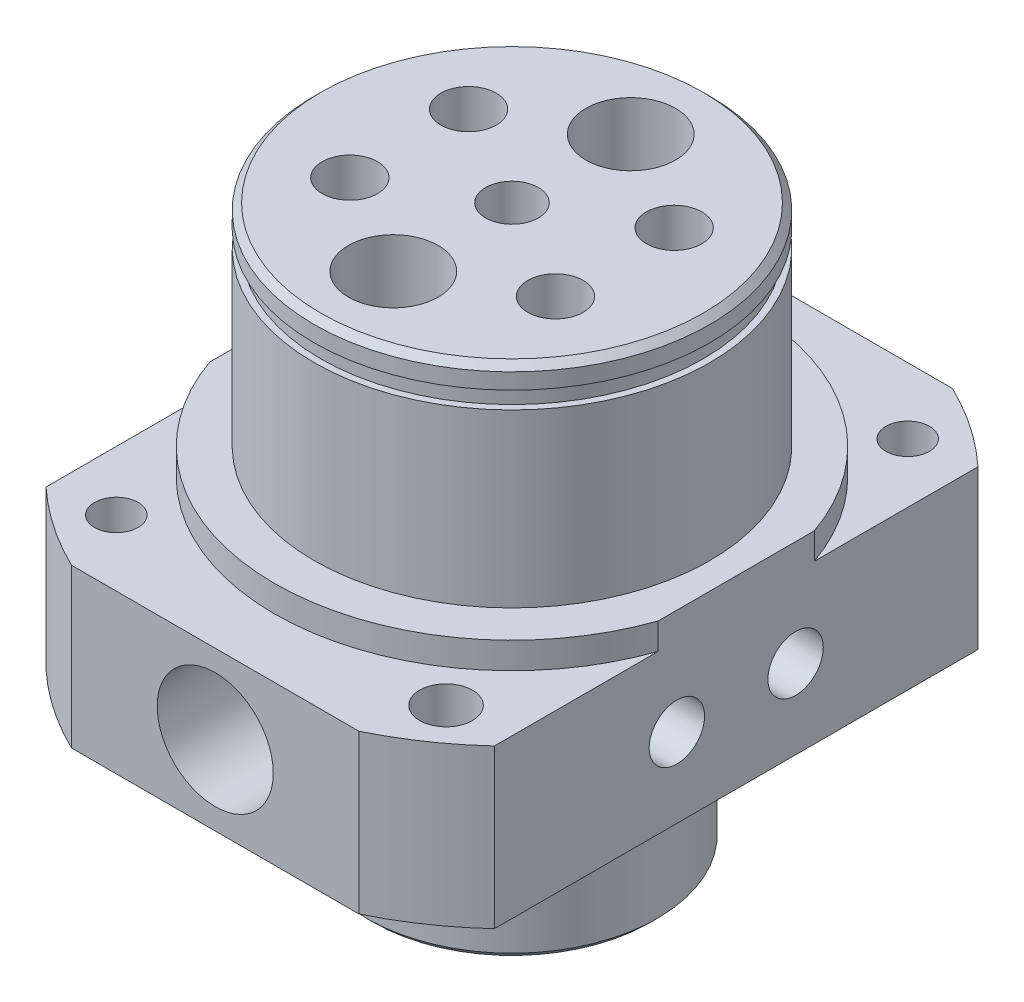
SolidWorks part; units mm, degrees
material "S45C"
ref_plane "Front Plane" through (0, 0, 0) normal (0, 0, 1) x (1, 0, 0)
ref_plane "Top Plane" through (0, 0, 0) normal (0, 1, 0) x (1, 0, 0)
ref_plane "Right Plane" through (0, 0, 0) normal (1, 0, 0) x (0, 0, -1)
sketch "Sketch1" plane through (0, 0, 0) normal (1, 0, 0) x (0, 0, -1)
  line L0 (0, 78.7622) -> (0, -44.4545) construction
  line L1 (0, -12) -> (11, -12)
  line L2 (11, -12) -> (11, 0)
  line L3 (11, 0) -> (25, 0)
  line L4 (25, 0) -> (25, 12)
  line L5 (25, 12) -> (18, 12)
  line L6 (15, 14) -> (15, 27)
  line L7 (15, 30) -> (0, 30)
  line L8 (0, 30) -> (0, -12)
  line L9 (18, 12) -> (18, 14)
  line L10 (18, 14) -> (15, 14)
  line L11 (15, 28.3) -> (14.5, 28.3)
  line L12 (14.5, 28.3) -> (14.5, 27)
  line L13 (14.5, 27) -> (15, 27)
  line L14 (15, 28.3) -> (15, 30)
  dimension "D1" = 11
  dimension "D2" = 25
  dimension "D3" = 15
  dimension "D4" = 12
  dimension "D5" = 12
  dimension "D6" = 13
  dimension "D7" = 18
  dimension "D8" = 2
  dimension "D9" = 14.5
  dimension "D10" = 1.3
  dimension "D11" = 1.7
revolve "Revolve1" add sketch "Sketch1" angle 360 about L0
sketch "Sketch2" plane through (0, 0, 0) normal (0, 1, 0) x (1, 0, 0)
  line L1 (-17, -22.5) -> (17, -22.5)
  line L2 (-17, -22.5) -> (-17, 22.5)
  line L3 (-17, 22.5) -> (17, 22.5)
  line L4 (17, -22.5) -> (17, 22.5)
  line L5 (-17, -22.5) -> (17, 22.5) construction
  line L6 (-17, 22.5) -> (17, -22.5) construction
  point P0 (0, 0)
  dimension "D1" = 34
  dimension "D2" = 45
extrude "Cut-Extrude1" cut sketch "Sketch2" along normal through all flip side to cut
sketch "Sketch3" plane through (0, -12, 0) normal (0, -1, 0) x (1, 0, 0)
  circle A0 centre (0, 0) radius 5.5
  dimension "D1" = 11
extrude "Cut-Extrude2" [suppressed] cut sketch "Sketch3" against normal through all
hole_wizard "M4 Tapped Hole1" positions "Sketch13" profile "Sketch12" tap size "M4" standard "Gb" end condition through all
sketch "Sketch13" plane through (0, 0, 0) normal (0, -1, 0) x (-1, 0, 0)
  line L1 (-12.5, -17.5) -> (12.5, -17.5) construction
  line L2 (-12.5, -17.5) -> (-12.5, 17.5) construction
  line L3 (-12.5, 17.5) -> (12.5, 17.5) construction
  line L4 (12.5, -17.5) -> (12.5, 17.5) construction
  line L5 (-12.5, -17.5) -> (12.5, 17.5) construction
  line L6 (-12.5, 17.5) -> (12.5, -17.5) construction
  point P0 (-12.5, 17.5)
  point P2 (12.5, -17.5)
  dimension "D1" = 35
  dimension "D2" = 25
sketch "Sketch12" plane through (12.5, 0, -17.5) normal (1, 0, 0) x (0, 0, -1)
  line L0 (0, 0) -> (0, 30)
  line L1 (0, 30) -> (1.65, 30)
  line L2 (1.65, 30) -> (1.65, 0)
  line L5 (1.65, 0) -> (0, 0)
  line L11 (0, -6.35) -> (0, 107.95) construction
  dimension "通孔螺纹孔钻头直径" = 3.3
  dimension "通孔螺纹孔钻头深度" = 30
cosmetic thread "Cosmetic Thread8" parameters "D2"=4
cosmetic thread "Cosmetic Thread11" parameters "D2"=4
sketch "Sketch14" plane through (0, 12, 0) normal (0, 1, 0) x (1, 0, 0)
  line L1 (12.5, -17.5) -> (-12.5, -17.5) construction
  line L2 (12.5, -17.5) -> (12.5, 17.5) construction
  line L3 (12.5, 17.5) -> (-12.5, 17.5) construction
  line L4 (-12.5, -17.5) -> (-12.5, 17.5) construction
  line L5 (12.5, -17.5) -> (-12.5, 17.5) construction
  line L6 (12.5, 17.5) -> (-12.5, -17.5) construction
  circle A0 centre (12.5, -17.5) radius 2
  circle A1 centre (-12.5, 17.5) radius 2
  point P2 (0, 0)
  dimension "D1" = 4
extrude "Cut-Extrude5" cut sketch "Sketch14" against normal through all
sketch "Sketch15" plane through (17, 0, 0) normal (1, 0, 0) x (0, 0, -1)
  line L0 (-3, 6) -> (3, 6) construction
  line L1 (-3, 9) -> (3, 9)
  line L2 (-3, 3) -> (3, 3)
  line L3 (22.5, 6) -> (-22.5, 6) construction
  line L4 (22.5, 12) -> (22.5, 0) construction
  line L5 (-22.5, 0) -> (-22.5, 12) construction
  arc A0 (-3, 9) -> (-3, 3) centre (-3, 6) ccw
  arc A1 (3, 3) -> (3, 9) centre (3, 6) ccw
  point P2 (0, 6)
  dimension "D2" = 3
  dimension "D1" = 6
extrude "Cut-Extrude6" [suppressed] cut sketch "Sketch15" against normal through all
sketch "Sketch17" plane through (0, 30, 0) normal (0, 1, 0) x (1, 0, 0)
  line L0 (0, -30.9464) -> (0, 32.404) construction
  line L1 (-7.7942, 4.5) -> (7.7942, -4.5) construction
  line L2 (7.7942, 4.5) -> (-7.7942, -4.5) construction
  circle A0 centre (-7.7942, 4.5) radius 2
  circle A1 centre (-7.7942, -4.5) radius 2
  circle A2 centre (0, -9) radius 3
  circle A3 centre (7.7942, 4.5) radius 2
  circle A4 centre (0, 9) radius 3
  circle A5 centre (7.7942, -4.5) radius 2
  circle A6 centre (0, 0) radius 2
  circle A7 centre (0, 0) radius 9 construction
  dimension "D1" = 6
  dimension "D2" = 4
  dimension "D3" = 4
  dimension "D4" = 18
  dimension "D5" = 60
  dimension "D6" = 60
extrude "Cut-Extrude7" cut sketch "Sketch17" against normal blind 28
sketch "Sketch18" plane through (-17, 0, 0) normal (-1, 0, 0) x (0, 0, 1)
  line L0 (0, 0) -> (0, 38.293) construction
  line L1 (-18.3303, 0) -> (18.3303, 0) construction
  circle A0 centre (-4.5, 6) radius 2
  circle A1 centre (4.5, 6) radius 2
  dimension "D1" = 9
  dimension "D2" = 6
  dimension "D3" = 4
extrude "Cut-Extrude10" cut sketch "Sketch18" against normal up to next
sketch "Sketch19" plane through (17, 0, 0) normal (1, 0, 0) x (0, 0, -1)
  circle A0 centre (-4.5, 6) radius 2
  circle A1 centre (4.5, 6) radius 2
  dimension "D1" = 4
extrude "Cut-Extrude11" cut sketch "Sketch19" against normal up to next
sketch "Sketch20" plane through (0, 0, -22.5) normal (0, 0, -1) x (-1, 0, 0)
  line L0 (-10.8972, 0) -> (10.8972, 0) construction
  circle A0 centre (0, 6) radius 3
  dimension "D1" = 6
  dimension "D2" = 6
extrude "Cut-Extrude12" cut sketch "Sketch20" against normal up to next
sketch "Sketch21" plane through (0, 0, 22.5) normal (0, 0, 1) x (1, 0, 0)
  circle A0 centre (0, 6) radius 3
  dimension "D1" = 6
extrude "Cut-Extrude13" cut sketch "Sketch21" against normal up to next
sketch "Sketch22" plane through (0, -12, 0) normal (0, -1, 0) x (1, 0, 0)
  circle A0 centre (0, 0) radius 2
  dimension "D1" = 4
extrude "Cut-Extrude14" cut sketch "Sketch22" against normal through all
chamfer "Chamfer1" distance 0.5 angle 45 2 edges at (0, -12, 11) (0, 30, 15)
chamfer "Chamfer2" [suppressed] distance 0.5 angle 45
hole_wizard "M8 Tapped Hole1" positions "Sketch24" profile "Sketch23" tap size "M8" standard "GB"
sketch "Sketch24" plane through (0, 30, 0) normal (0, 1, 0) x (1, 0, 0)
  point P0 (0, 9)
  point P3 (0, -9)
sketch "Sketch23" plane through (0, 30, -9) normal (1, 0, 0) x (0, 0, 1)
  line L0 (0, 0) -> (0, 17.0429)
  line L1 (0, 17.0429) -> (3.4, 15)
  line L2 (3.4, 15) -> (3.4, 0)
  line L5 (3.4, 0) -> (0, 0)
  line L10 (0, 17.0429) -> (-3.4, 15) construction
  line L11 (0, -6.35) -> (0, 107.95) construction
  dimension "螺纹孔钻头直径" = 6.8
  dimension "螺纹孔钻头深度" = 15
  dimension "导头角度" = 118
cosmetic thread "Cosmetic Thread12" parameters "D1"=15, "D2"=8
cosmetic thread "Cosmetic Thread13" parameters "D1"=15, "D2"=8
hole_wizard "M5 Tapped Hole2" positions "Sketch26" profile "Sketch25" tap size "M5" standard "GB"
sketch "Sketch26" plane through (0, 30, 0) normal (0, 1, 0) x (1, 0, 0)
  point P0 (7.7942, 4.5)
  point P3 (7.7942, -4.5)
  point P6 (-7.7942, -4.5)
  point P9 (-7.7942, 4.5)
sketch "Sketch25" plane through (7.7942, 30, -4.5) normal (1, 0, 0) x (0, 0, 1)
  line L0 (0, 0) -> (0, 13.2618)
  line L1 (0, 13.2618) -> (2.1, 12)
  line L2 (2.1, 12) -> (2.1, 0)
  line L5 (2.1, 0) -> (0, 0)
  line L10 (0, 13.2618) -> (-2.1, 12) construction
  line L11 (0, -6.35) -> (0, 107.95) construction
  dimension "螺纹孔钻头直径" = 4.2
  dimension "螺纹孔钻头深度" = 12
  dimension "导头角度" = 118
cosmetic thread "Cosmetic Thread14" parameters "D1"=10, "D2"=5
cosmetic thread "Cosmetic Thread15" parameters "D1"=10, "D2"=5
cosmetic thread "Cosmetic Thread16" parameters "D1"=10, "D2"=5
cosmetic thread "Cosmetic Thread17" parameters "D1"=10, "D2"=5
hole_wizard "M5 Tapped Hole1" positions "Sketch28" profile "Sketch27" tap size "M5" standard "GB"
sketch "Sketch28" plane through (-17, 0, 0) normal (-1, 0, 0) x (0, 0, 1)
  point P0 (-4.5, 6)
  point P3 (4.5, 6)
cosmetic thread "Cosmetic Thread18" parameters "D1"=10, "D2"=5
cosmetic thread "Cosmetic Thread19" parameters "D1"=10, "D2"=5
sketch "Sketch27" plane through (-17, 6, -4.5) normal (0, 1, 0) x (0, 0, 1)
  line L0 (0, 0) -> (0, 13.2618)
  line L1 (0, 13.2618) -> (2.1, 12)
  line L2 (2.1, 12) -> (2.1, 0)
  line L5 (2.1, 0) -> (0, 0)
  line L10 (0, 13.2618) -> (-2.1, 12) construction
  line L11 (0, -6.35) -> (0, 107.95) construction
  dimension "螺纹孔钻头直径" = 4.2
  dimension "螺纹孔钻头深度" = 12
  dimension "导头角度" = 118
hole_wizard "M5 Tapped Hole3" positions "Sketch30" profile "Sketch29" tap size "M5" standard "GB"
sketch "Sketch30" plane through (17, 0, 0) normal (1, 0, 0) x (0, 0, -1)
  point P0 (4.5, 6)
  point P3 (-4.5, 6)
sketch "Sketch29" plane through (17, 6, -4.5) normal (0, 1, 0) x (0, 0, -1)
  line L0 (0, 0) -> (0, 13.2618)
  line L1 (0, 13.2618) -> (2.1, 12)
  line L2 (2.1, 12) -> (2.1, 0)
  line L5 (2.1, 0) -> (0, 0)
  line L10 (0, 13.2618) -> (-2.1, 12) construction
  line L11 (0, -6.35) -> (0, 107.95) construction
  dimension "螺纹孔钻头直径" = 4.2
  dimension "螺纹孔钻头深度" = 12
  dimension "导头角度" = 118
cosmetic thread "Cosmetic Thread20" parameters "D1"=10, "D2"=5
cosmetic thread "Cosmetic Thread21" parameters "D1"=10, "D2"=5
hole_wizard "G1/8 Tapped Hole1" positions "Sketch32" profile "Sketch31" tap size "G1/8" standard "GB"
sketch "Sketch32" plane through (0, 0, 22.5) normal (0, 0, 1) x (1, 0, 0)
  point P0 (0, 6)
sketch "Sketch31" plane through (0, 6, 22.5) normal (1, 0, 0) x (0, -1, 0)
  line L0 (0, 0) -> (0, 17.6438)
  line L1 (0, 17.6438) -> (4.4, 15)
  line L2 (4.4, 15) -> (4.4, 0)
  line L5 (4.4, 0) -> (0, 0)
  line L10 (0, 17.6438) -> (-4.4, 15) construction
  line L11 (0, -6.35) -> (0, 107.95) construction
  dimension "螺纹孔钻头直径" = 8.8
  dimension "螺纹孔钻头深度" = 15
  dimension "导头角度" = 118
cosmetic thread "Cosmetic Thread22" parameters "D1"=15, "D2"=9.728
hole_wizard "G1/8 Tapped Hole2" positions "Sketch34" profile "Sketch33" tap size "G1/8" standard "GB"
sketch "Sketch34" plane through (0, 0, -22.5) normal (0, 0, -1) x (-1, 0, 0)
  point P0 (0, 6)
sketch "Sketch33" plane through (0, 6, -22.5) normal (1, 0, 0) x (0, 1, 0)
  line L0 (0, 0) -> (0, 17.6438)
  line L1 (0, 17.6438) -> (4.4, 15)
  line L2 (4.4, 15) -> (4.4, 0)
  line L5 (4.4, 0) -> (0, 0)
  line L10 (0, 17.6438) -> (-4.4, 15) construction
  line L11 (0, -6.35) -> (0, 107.95) construction
  dimension "螺纹孔钻头直径" = 8.8
  dimension "螺纹孔钻头深度" = 15
  dimension "导头角度" = 118
cosmetic thread "Cosmetic Thread23" parameters "D1"=15, "D2"=9.728
